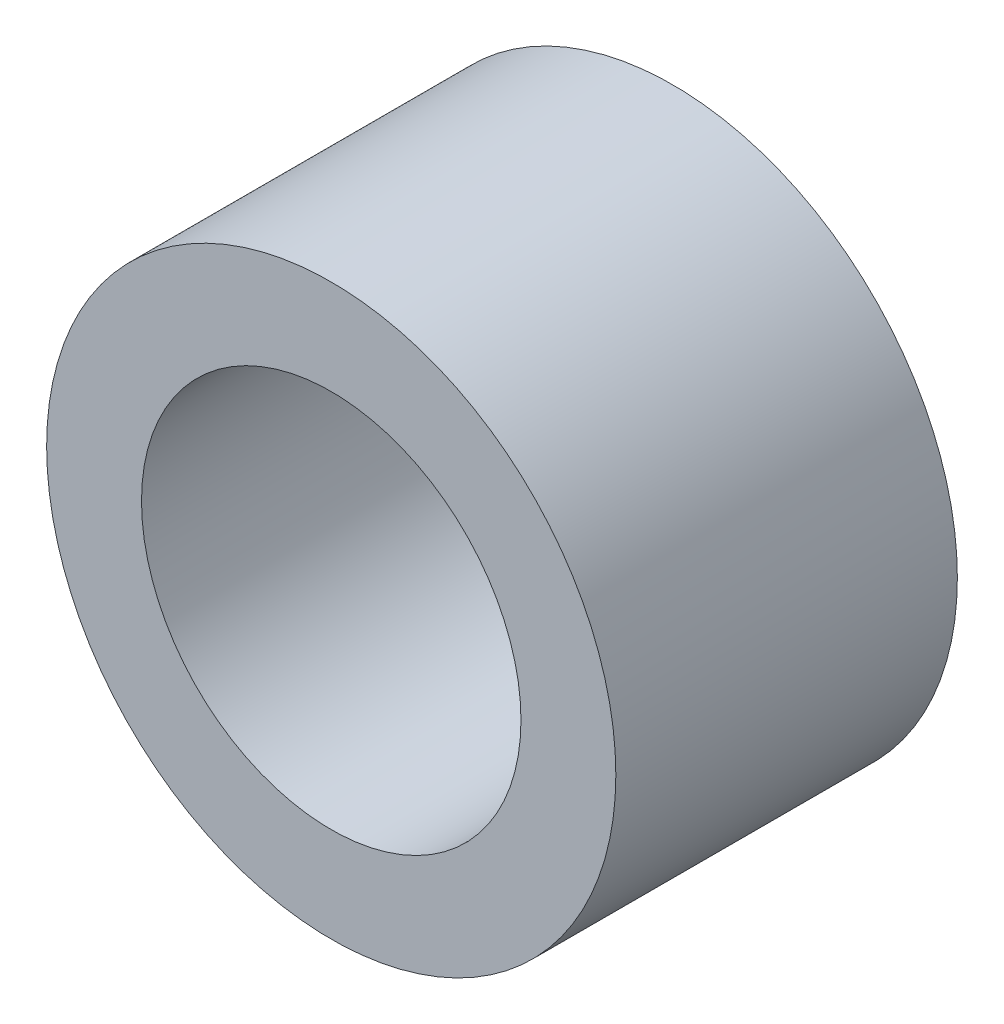
SolidWorks part; units mm, degrees
material "6061 合金"
ref_plane "Front Plane" through (0, 0, 0) normal (0, 0, 1) x (1, 0, 0)
ref_plane "Top Plane" through (0, 0, 0) normal (0, 1, 0) x (1, 0, 0)
ref_plane "Right Plane" through (0, 0, 0) normal (1, 0, 0) x (0, 0, -1)
sketch "Sketch1" plane through (0, 0, 0) normal (0, 0, 1) x (1, 0, 0)
  circle A0 centre (0, 0) radius 7.5
  circle A1 centre (0, 0) radius 5
  dimension "D1" = 15
  dimension "D2" = 10
extrude "Boss-Extrude1" add sketch "Sketch1" along normal blind 9
